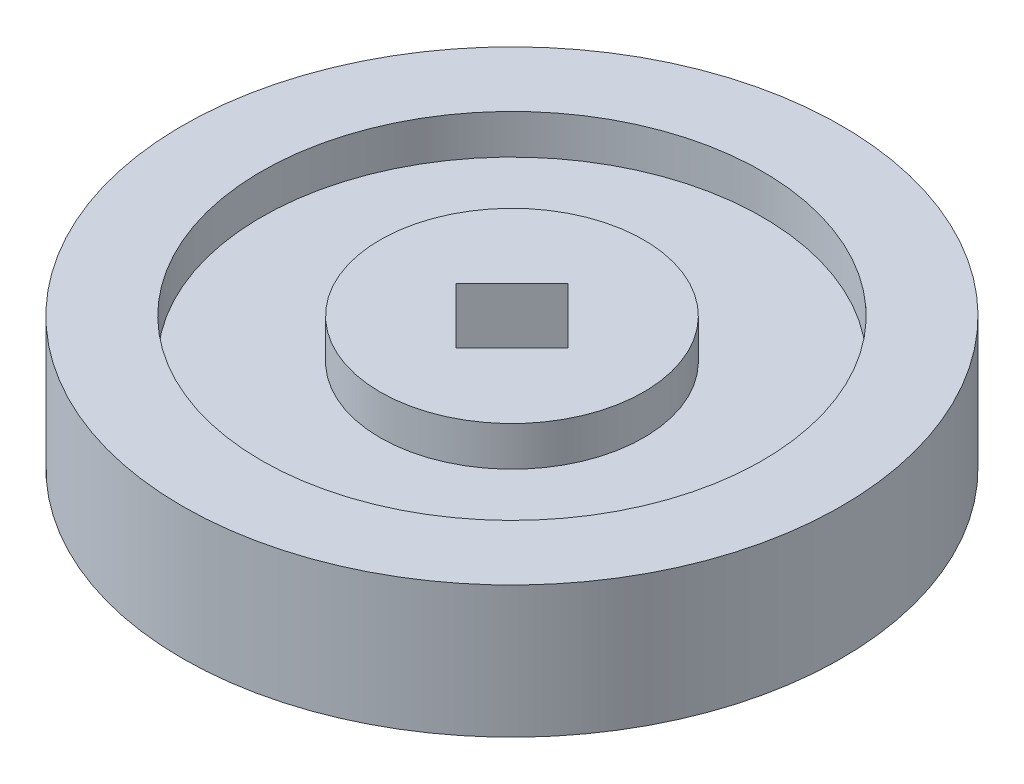
SolidWorks part; units mm, degrees
ref_plane "Front Plane" through (0, 0, 0) normal (0, 0, 1) x (1, 0, 0)
ref_plane "Top Plane" through (0, 0, 0) normal (0, 1, 0) x (1, 0, 0)
ref_plane "Right Plane" through (0, 0, 0) normal (1, 0, 0) x (0, 0, -1)
other "Configuration Table"
sketch "Sketch1" plane through (0, 0, 0) normal (0, 1, 0) x (1, 0, 0)
  circle A0 centre (0, 0) radius 25
  circle A1 centre (0, 0) radius 19
  dimension "D1" = 50
  dimension "D2" = 38
extrude "Boss-Extrude1" add sketch "Sketch1" along normal mid plane 10
sketch "Sketch2" plane through (0, 5, 0) normal (0, 1, 0) x (1, 0, 0)
  circle A1 centre (0, 0) radius 10
  dimension "D1" = 20
extrude "Boss-Extrude2" add sketch "Sketch2" against normal blind 12 separate body
sketch "Sketch3" plane through (0, 0, 0) normal (0, 1, 0) x (1, 0, 0)
  circle A0 centre (0, 0) radius 19 construction
  circle A1 centre (0, 0) radius 10
  circle A2 centre (0, 0) radius 10
  circle A3 centre (0, 0) radius 19
  dimension "D1" = 0
extrude "Boss-Extrude3" add sketch "Sketch3" along normal mid plane 4
sketch "Sketch4" plane through (0, -7, 0) normal (0, -1, 0) x (1, 0, 0)
  line L0 (-4.2426, 0) -> (0, 4.2426)
  line L1 (-4.2426, 0) -> (0, -4.2426)
  line L2 (0, 4.2426) -> (4.2426, 0)
  line L3 (0, -4.2426) -> (4.2426, 0)
  line L4 (-4.2426, 0) -> (4.2426, 0) construction
  line L5 (0, 4.2426) -> (0, -4.2426) construction
  point P1 (0, 0)
  dimension "D1" = 6
extrude "Cut-Extrude1" cut sketch "Sketch4" against normal blind 50
